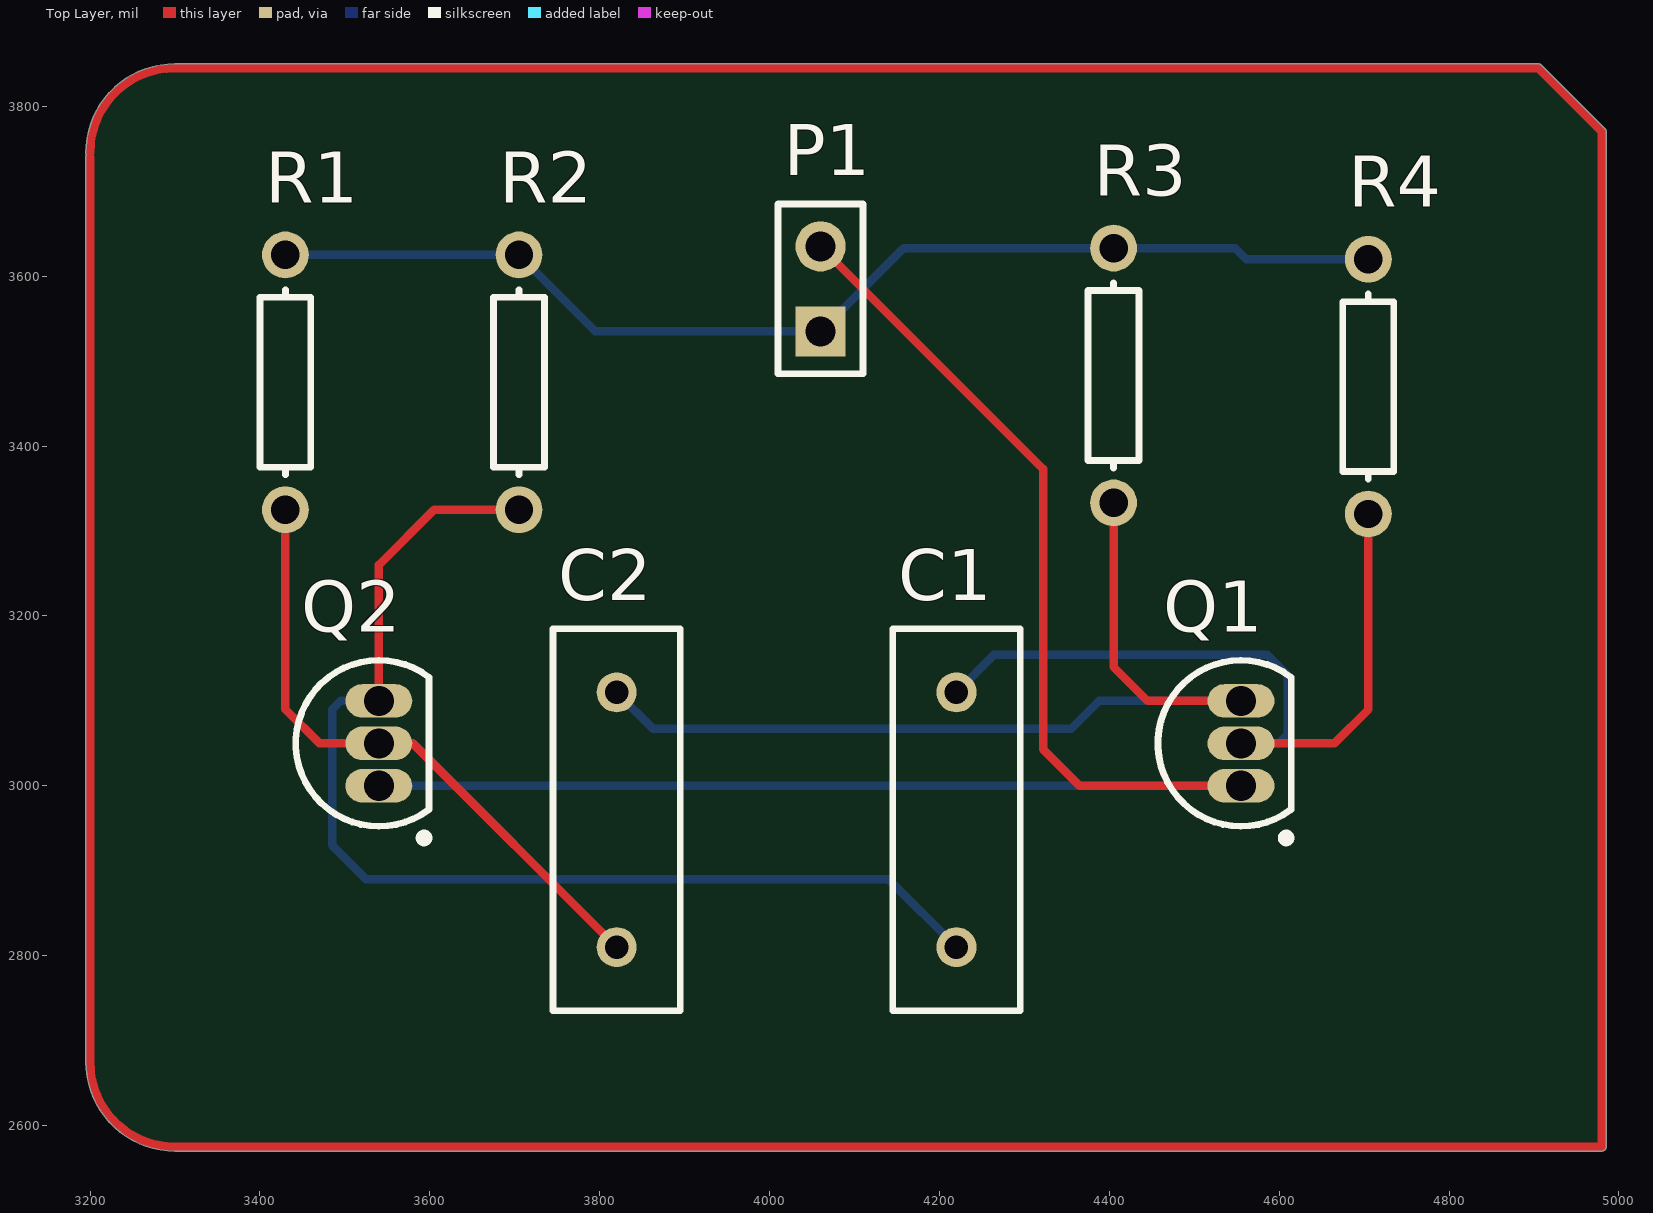
[diagram p0: Top Layer view]
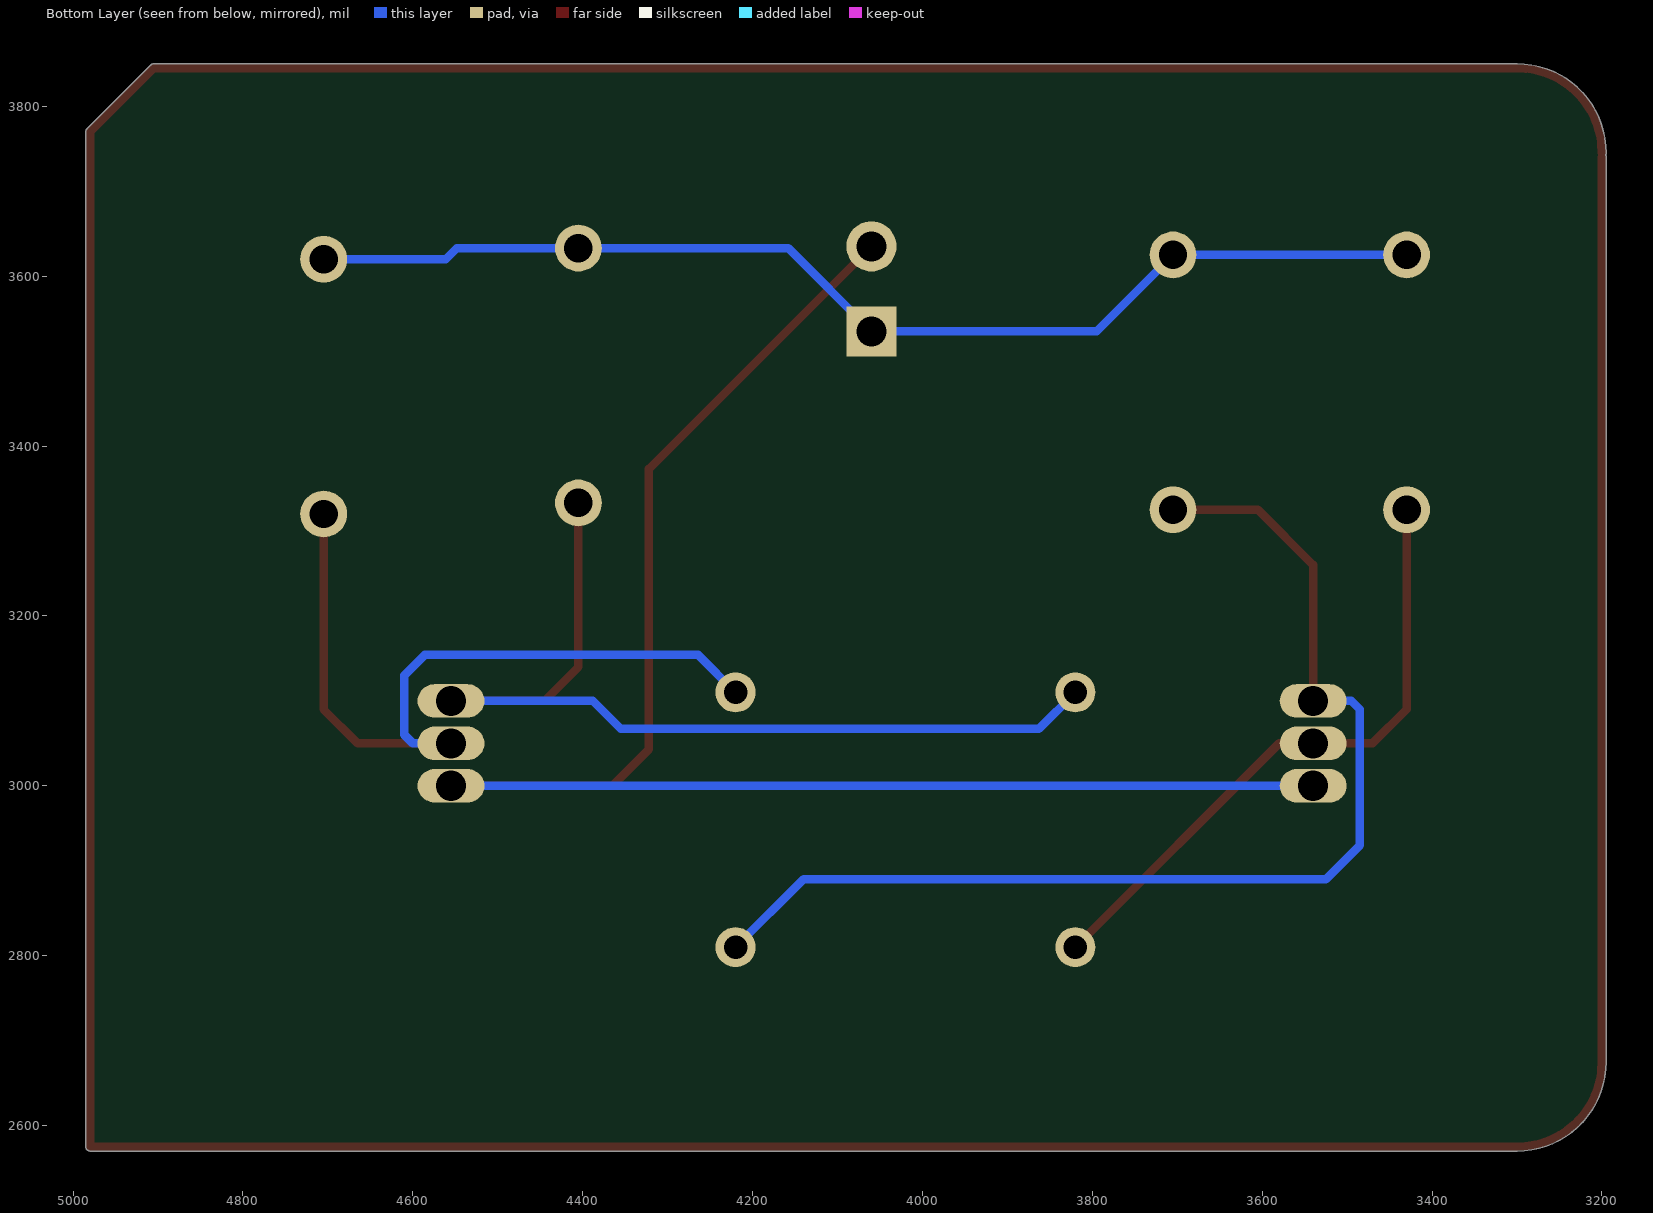
[diagram p1: Bottom Layer view, seen from below]
# Altium PCB MISC80684-6.PcbDoc
Units mil, origin at the board's own origin, x right, y up, seen from the top; angles counter-clockwise.
Board outline 1790.03 x 1280.03 mil, 2 copper layers (Top Layer, Bottom Layer); 9 components, 0 nets, 20 pads, 0 vias.

## Layer stack, top to bottom (the 12.6 mil dielectric is the usual default, probably not edited)
Top Solder: solder mask 0.4, Solder Resist, Dk 3.5
Top Layer: signal copper 1.4
Dielectric 1: dielectric 12.6, FR-4, Dk 4.8
Bottom Layer: signal copper 1.4
Bottom Solder: solder mask 0.4, Solder Resist, Dk 3.5

## Board outline
3194.99,2675 3194.99,3740 cw(c3200,3740) 3195.65,3742.5 cw(c3200,3745) 3194.99,3745 cw(c3300,3745) 3300,3850.01 4905,3850.01 cw(c4905,3845) 4908.56,3848.53 4908.55,3848.55 4983.55,3773.55 4983.53,3773.56 cw(c4980,3770) 4985.02,3770 4985.02,2575 cw(c4980,2575) 4980,2569.99 3300,2569.99 cw(c3300,2675)

## Design rules (kind name [scope] priority, off if disabled: settings)
Clearance [All] p1: gap=10
PolygonConnect [All] p1: connectstyle=Relief reliefconductorwidth=10 reliefentries=4 polygonreliefangle="90 Angle" airgapwidth=10
RoutingVias [All] p1: holewidth=28 width=50 viastyle="Through Hole" minholewidth=28 minwidth=50 maxholewidth=28 maxwidth=50
SolderMaskExpansion [All] p1: expansion=4
Width [All] p1: maxlimit=10 minlimit=10 preferedwidth=10
30 further rules are at their usual default settings.

## Components (designator, comment, footprint, x,y, rotation, side; value= is the part's Value field where it differs from the comment)
C1 "Cap" RAD-0.3 4220,2960 r90 top
C2 "Cap" RAD-0.3 3820,2960 r90 top
P1 "Header 2" HDR1X2 4060,3535 r90 top
Q1 "2N3904" TO-92A 4555,3050 r0 top
Q2 "2N3904" TO-92A 3540,3050 r0 top
R1 "Res1" AXIAL-0.3 3430,3475 r90 top
R2 "Res1" AXIAL-0.3 3705,3475 r90 top
R3 "Res1" AXIAL-0.3 4405,3483.03 r90 top
R4 "Res1" AXIAL-0.3 4705,3470 r90 top

## Footprints (in the part's own frame and the unit in brackets; to place one, negate y for a bottom-side part, rotate by r counter-clockwise, add the part's x,y. Pads: shape width x height; smd on the part's side, far side on the other; paste and mask are expansions set on the pad)
AXIAL-0.3 [mm] "Axial Device, Thru-Hole; 2 Leads; 0.3 in Pin Spacing"
  round 1.4 hole 0.85: 1(-3.81,0) 2(3.81,0)
  silkscreen extent -2.77,-0.76 2.77,0.76
HDR1X2 [mm] "Connector; Header; 2 Position"
  rect 1.5x1.5 hole 0.9: 1(0,0)
  round 1.5 hole 0.9: 2(2.54,0)
  silkscreen extent -1.27,-1.27 3.81,1.27
RAD-0.3 [mm] "Radial Cap, Thru-Hole; 2 Leads; 0.3 in Pin Spacing"
  round 1.2 hole 0.7: 1(-3.81,0) 2(3.81,0)
  silkscreen extent -5.71,-1.91 5.71,1.91
TO-92A [mm] "TO, Flat Index; 3 In-Line, Axial Leads; Body Dia. 4.5mm; Leads 0.51 x 0.48 mm (max)"
  oval 2x1 hole 0.9: 1(0,-1.27) 2(0,0) 3(0,1.27)
  silkscreen extent -2.48,-2.95 1.5,2.48, body extent -2.48,-2.5 1.5,2.5, height 6.86

## Part data
C1 C2: "Capacitor"
P1: "Header, 2-Pin"
Q1 Q2: "NPN General Purpose Amplifier"
R1 R2 R3 R4: "Resistor"

## Nets (pads, with @x,y where several pads share a name; then routed paths per layer and width w, separated by ;. In a path a pad name is that pad's centre, name@x,y a point inside that pad or via, vN(x,y) a via of type N, cw(c..) or ccw(c..) an arc to the next point about the centre after c; other vN are vias at no path point)
pads on no net: C1.1 C1.2 C2.1 C2.2 P1.1 P1.2 Q1.1 Q1.2 Q1.3 Q2.1 Q2.2 Q2.3 R1.1 R1.2 R2.1 R2.2 R3.1 R3.2 R4.1 R4.2
copper on no net: | length 13506.6
  Top Layer w10: 3200,3740 3200,2675 ccw(c3300,2675) 3300,2575 3310,2575 4980,2575 4980,3770 4905,3845 3325,3845 ; 3200,3745 cw(c3300,3745) 3300,3845 3305,3845 3325,3845 ; 3375,3845 3325,3845 ; 3430,3325 3430,3090 3470,3050 3540,3050 3580,3050 3820,2810 ; 3540,3100 3540,3260 3605,3325 3705,3325 ; 4060,3635 4322,3373 4322,3043 4365,3000 4555,3000 ; 4405,3333.03 4405,3140 4445,3100 4555,3100 ; 4555,3050 4665,3050 4705,3090 4705,3320
  Bottom Layer w10: 3430,3625 3705,3625 3795,3535 4060,3535 4158.03,3633.03 4405,3633.03 4548,3633.03 4561.03,3620 4705,3620 ; 3540,3000 4555,3000 ; 3540,3100 3495,3100 3485,3090 3485,2930 3525,2890 4140,2890 4220,2810 ; 3820,3110 3863,3067 4355,3067 4388,3100 4555,3100 ; 4220,3110 4264,3154 4586,3154 4610,3130 4610,3060 4600,3050 4555,3050